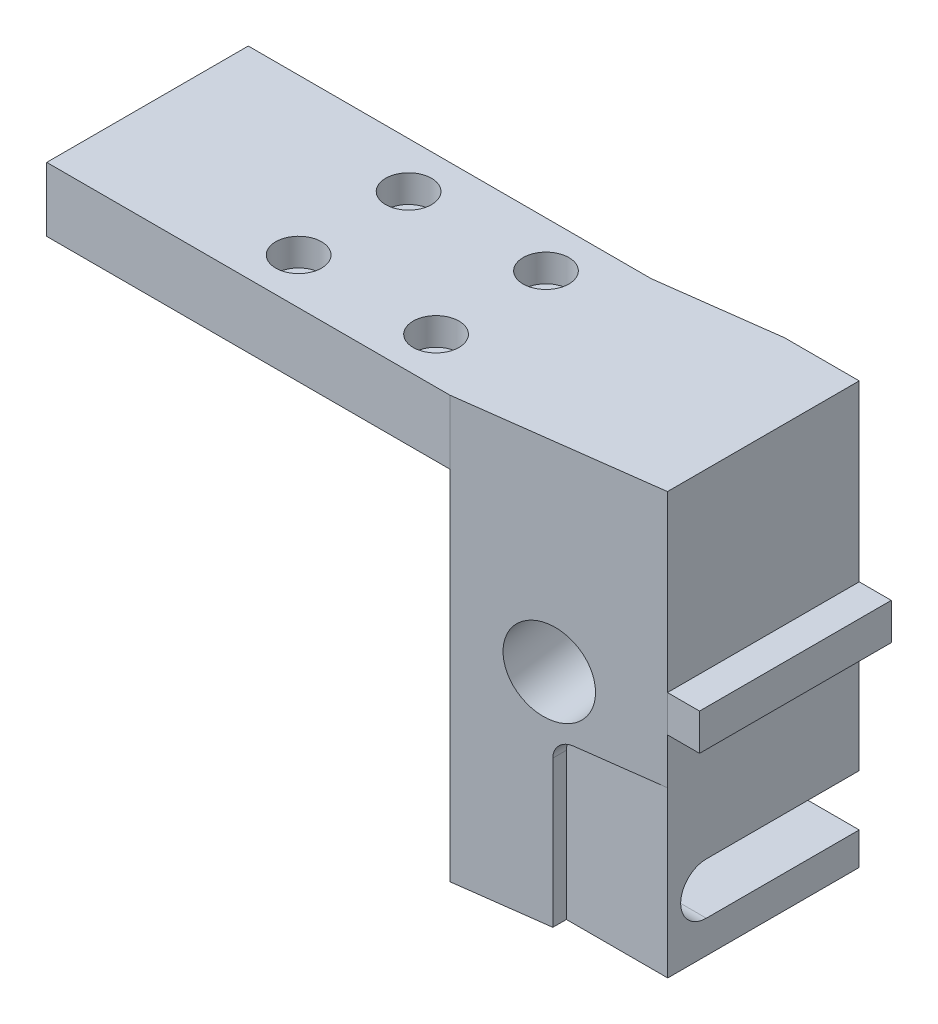
SolidWorks part; units mm, degrees
material "6061 合金"
ref_plane "前视基准面" through (0, 0, 0) normal (0, 0, 1) x (1, 0, 0)
ref_plane "上视基准面" through (0, 0, 0) normal (0, 1, 0) x (1, 0, 0)
ref_plane "右视基准面" through (0, 0, 0) normal (1, 0, 0) x (0, 0, -1)
sketch "草图1" plane through (0, 0, 0) normal (0, 0, 1) x (1, 0, 0)
  line L0 (30.6322, 5.3659) -> (34.1322, 5.3659)
  line L1 (-34.3678, 24.3659) -> (30.6322, 24.3659)
  line L2 (-34.3678, 24.3659) -> (-34.3678, -21.6341)
  line L3 (-34.3678, -21.6341) -> (30.6322, -21.6341)
  line L4 (30.6322, 24.3659) -> (30.6322, 5.3659)
  line L5 (34.1322, 5.3659) -> (34.1322, 1.3659)
  line L6 (34.1322, 1.3659) -> (30.6322, 1.3659)
  line L7 (30.6322, 1.3659) -> (30.6322, -21.6341)
  dimension "D1" = 46
  dimension "D2" = 65
  dimension "D3" = 19
  dimension "D4" = 3.5
  dimension "D5" = 4
extrude "凸台-拉伸1" add sketch "草图1" along normal blind 23.69
sketch "草图2" plane through (0, 0, 0) normal (0, 0, -1) x (-1, 0, 0)
  line L1 (34.3678, -21.6341) -> (-9.6322, -21.6341)
  line L2 (34.3678, -21.6341) -> (34.3678, 17.3659)
  line L3 (34.3678, 17.3659) -> (-9.6322, 17.3659)
  line L4 (-9.6322, -21.6341) -> (-9.6322, 17.3659)
  dimension "D1" = 44
  dimension "D2" = 39
extrude "切除-拉伸1" cut sketch "草图2" against normal up to next
sketch "草图3" plane through (30.6322, 0, 0) normal (1, 0, 0) x (0, 0, -1)
  line L0 (0, -21.6341) -> (0, 1.3659) construction
  line L2 (0, -18.0845) -> (0, -12.4845)
  line L3 (0, -12.4845) -> (-16.69, -12.4845)
  line L5 (0, -18.0845) -> (-16.69, -18.0845)
  arc A1 (-16.69, -12.4845) -> (-16.69, -18.0845) centre (-16.69, -15.2845) ccw
  dimension "D1" = 16.69
  dimension "D2" = 5.6
extrude "切除-拉伸2" cut sketch "草图3" against normal up to next
sketch "草图4" plane through (0, 24.3659, 0) normal (0, 1, 0) x (1, 0, 0)
  line L0 (9.6322, -23.69) -> (34.1322, -23.69)
  line L1 (30.6322, -23.69) -> (-34.3678, -23.69) construction
  line L2 (34.1322, -23.69) -> (34.1322, -20.93)
  line L3 (34.1322, -23.69) -> (34.1322, 0) construction
  line L4 (34.1322, -20.93) -> (30.6322, -20.93)
  line L5 (30.6322, -23.69) -> (30.6322, 0) construction
  line L6 (30.6322, -20.93) -> (9.6322, -23.69)
  line L7 (-34.3678, -1.69) -> (-34.3678, 0)
  line L8 (-34.3678, -23.69) -> (-34.3678, 0) construction
  line L9 (-34.3678, 0) -> (22.4822, 0)
  line L10 (30.6322, 0) -> (-34.3678, 0) construction
  line L11 (22.4822, 0) -> (9.6322, -1.69)
  line L12 (9.6322, -1.69) -> (-34.3678, -1.69)
  dimension "D1" = 24.5
  dimension "D2" = 2.76
  dimension "D3" = 56.85
  dimension "D4" = 44
  dimension "D5" = 1.69
extrude "切除-拉伸3" cut sketch "草图4" against normal through all
sketch "草图5" plane through (0, 0, 23.69) normal (0, 0, 1) x (1, 0, 0)
  line L2 (30.6322, -21.6341) -> (19.5722, -21.6341)
  line L4 (30.6322, -21.6341) -> (30.6322, -3.6341)
  line L5 (30.6322, -3.6341) -> (21.5722, -3.6341)
  line L6 (19.5722, -21.6341) -> (19.5722, -5.6341)
  arc A0 (21.5722, -3.6341) -> (19.5722, -5.6341) centre (21.5722, -5.6341) ccw
  dimension "D1" = 18
  dimension "D2" = 11.06
  dimension "D3" = 2
extrude "切除-拉伸4" cut sketch "草图5" against normal blind 2.79
sketch "草图7" plane through (3.2242, 0, 24.5322) normal (0.1303, 0, 0.9915) x (0.9915, 0, -0.1303)
  line L0 (27.6437, 24.3659) -> (6.4631, 24.3659) construction
  line L1 (6.4631, 17.3659) -> (6.4631, -21.6341) construction
  circle A0 centre (16.1431, 2.3659) radius 4.5
  dimension "D1" = 9
  dimension "D2" = 22
  dimension "D3" = 9.68
extrude "切除-拉伸5" cut sketch "草图7" against normal up to next
sketch "草图8" plane through (-34.3678, 0, 0) normal (-1, 0, 0) x (0, 0, 1)
  line L0 (23.69, 24.3659) -> (1.69, 24.3659) construction
  line L1 (1.69, 17.3659) -> (1.69, 24.3659) construction
  line L2 (23.69, 24.3659) -> (23.69, 17.3659) construction
  circle A0 centre (7.69, 20.8659) radius 1.25
  circle A1 centre (17.69, 20.8659) radius 1.25
  dimension "D1" = 2.5
  dimension "D4" = 2.5
  dimension "D2" = 3.5
  dimension "D3" = 6
  dimension "D5" = 6
  dimension "D6" = 3.5
extrude "切除-拉伸6" cut sketch "草图8" against normal blind 8.5
sketch "草图10" plane through (0, 24.3659, 0) normal (0, 1, 0) x (1, 0, 0)
  line L0 (-34.3678, -23.69) -> (-34.3678, -1.69) construction
  line L1 (9.6322, -23.69) -> (-34.3678, -23.69) construction
  line L2 (-34.3678, -1.69) -> (9.6322, -1.69) construction
  circle A0 centre (-11.8678, -18.69) radius 1.45
  circle A1 centre (-11.8678, -6.69) radius 1.45
  circle A2 centre (3.1322, -18.69) radius 1.45
  circle A3 centre (3.1322, -6.69) radius 1.45
  dimension "D1" = 2.9
  dimension "D2" = 2.9
  dimension "D3" = 2.9
  dimension "D4" = 2.9
  dimension "D5" = 22.5
  dimension "D6" = 5
  dimension "D7" = 5
  dimension "D8" = 22.5
  dimension "D9" = 5
  dimension "D10" = 5
  dimension "D11" = 15
  dimension "D12" = 15
extrude "切除-拉伸7" cut sketch "草图10" against normal through all
sketch "草图11" plane through (0, 24.3659, 0) normal (0, 1, 0) x (1, 0, 0)
  circle A0 centre (-11.8678, -6.69) radius 2.5
  circle A1 centre (-11.8678, -18.69) radius 2.5
  circle A2 centre (3.1322, -6.69) radius 2.5
  circle A3 centre (3.1322, -18.69) radius 2.5
  dimension "D1" = 5
  dimension "D2" = 5
  dimension "D3" = 5
  dimension "D4" = 5
extrude "切除-拉伸8" cut sketch "草图11" against normal blind 3
sketch "草图12" plane through (0, 0, 0) normal (0, 0, -1) x (-1, 0, 0)
  line L0 (-30.6322, 5.3659) -> (-30.6322, 24.3659) construction
  line L1 (-30.6322, 24.3659) -> (-22.4822, 24.3659) construction
  circle A0 centre (-26.6322, 20.1159) radius 2.25
  dimension "D1" = 4.5
  dimension "D2" = 4
  dimension "D3" = 4.25
extrude "切除-拉伸9" cut sketch "草图12" against normal blind 6
